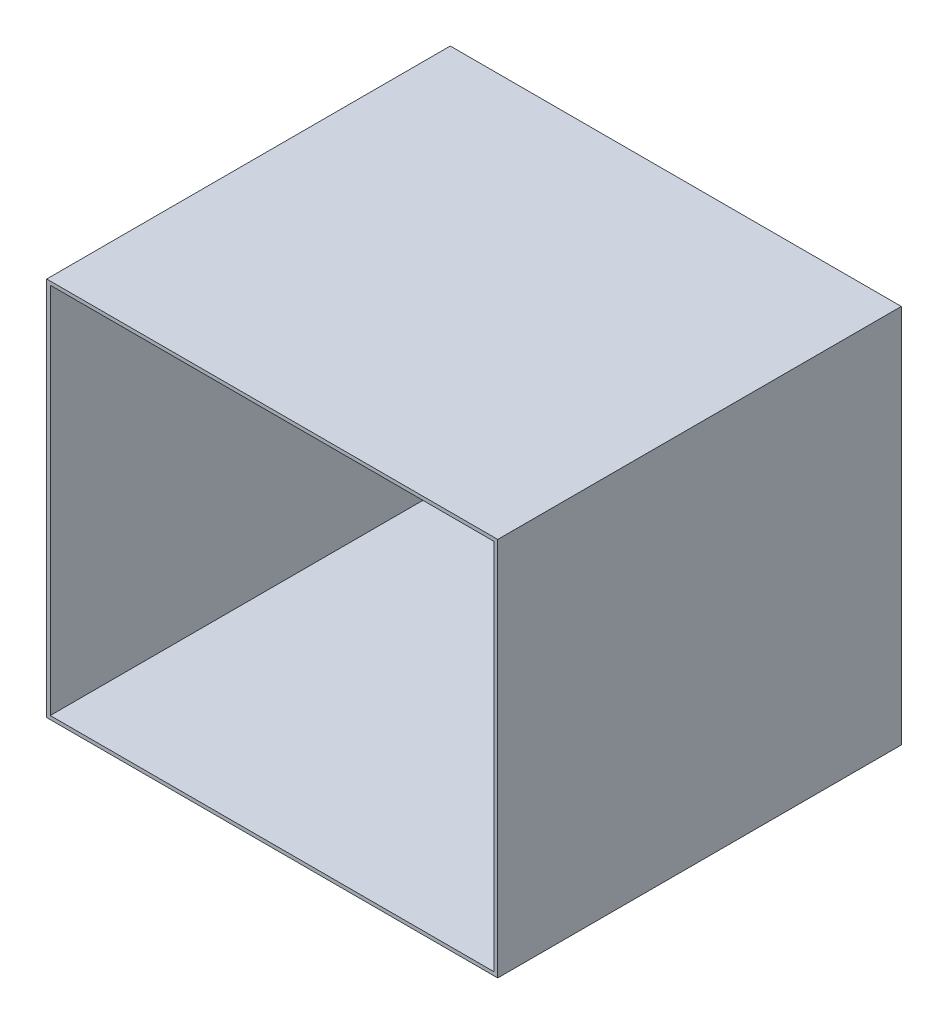
from build123d import *

# Parameters (mm, degrees)
SKETCH_1_W      = 380
SKETCH_1_H      = 320
SKETCH_1_W_2    = 374
SKETCH_1_H_2    = 314
EXTRUDE_1_DEPTH = 170


with BuildPart() as part:
    # 草图1 → 凸台-拉伸1 (new, symmetric)
    with BuildSketch(Plane.XY):
        Rectangle(SKETCH_1_W, SKETCH_1_H)
        Rectangle(SKETCH_1_W_2, SKETCH_1_H_2, mode=Mode.SUBTRACT)
    extrude(amount=EXTRUDE_1_DEPTH, both=True)


solid = part.part
